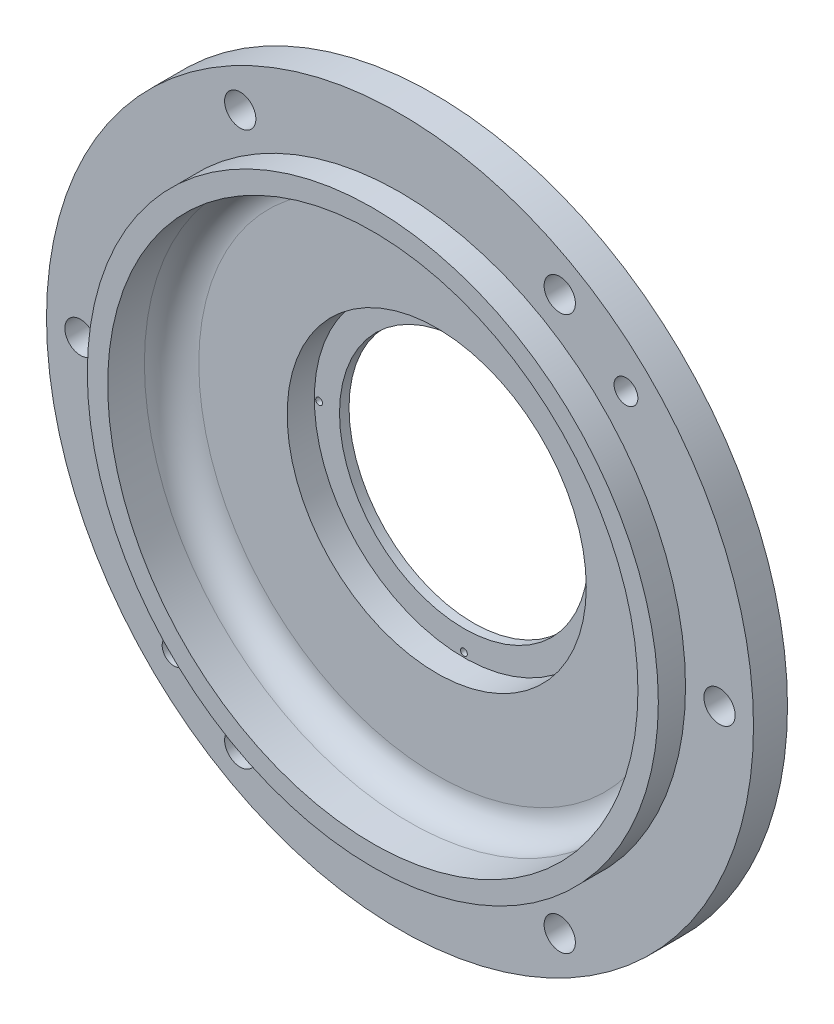
from build123d import *

# Parameters (mm, degrees)
FILLET1_R          = 20
CUT_EXTRUDE1_REACH = 377.068
SKETCH2_R          = 2.5
CIRPATTERN1_COUNT  = 4
CUT_EXTRUDE2_START = -372.639610375
SKETCH3_R          = 11.5
CUT_EXTRUDE2_DEPTH = 377.639610375
CIRPATTERN2_COUNT  = 6
M20_TAPPED_HOLE1_D = 17.5
CIRPATTERN3_COUNT  = 2


with BuildPart() as part:
    # Sketch1 → Revolve1 (revolve)
    with BuildSketch(Plane(origin=(0, 0, 0), x_dir=(0, 0, -1), z_dir=(1, 0, 0)), mode=Mode.PRIVATE) as revolve1_sk:
        Polygon((0, 260), (25, 260), (25, 210), (29.751288694, 210), (54, 168), (54, 91.5), (47, 91.5), (47, 110), (27, 110), (27, 195), (-20, 195), (-20, 210), (0, 210), align=None)
    revolve(revolve1_sk.sketch.rotate(Axis((0, 0, 141.233138436), (0, 0, -1)), 90), axis=Axis((0, 0, 141.233138436), (0, 0, -1)))

    # Fillet1
    fillet1_edges = [part.edges().sort_by_distance(p)[0] for p in [
        (-195, 0, -27),
    ]]
    fillet(fillet1_edges, radius=FILLET1_R)

    # Sketch2 → Cut-Extrude1 (cut, up to next)
    with BuildSketch(Plane(origin=(0, 0, -54), x_dir=(-1, 0, 0), z_dir=(0, 0, -1)), mode=Mode.PRIVATE) as cut_extrude1_sk1:
        with Locations((0, 106.5)):
            Circle(SKETCH2_R)
    cut_extrude1_tool1 = extrude(cut_extrude1_sk1.sketch, amount=-CUT_EXTRUDE1_REACH, mode=Mode.PRIVATE) & part.part
    cut_extrude1 = cut_extrude1_tool1.solids().sort_by_distance((0, 106.5, -54))[0]
    add(cut_extrude1, mode=Mode.SUBTRACT)

    # CirPattern1: Cut-Extrude1 ×4 about axis
    cirpattern1_axis = Axis((0, 0, 0), (0, 0, 1))
    for i in range(1, CIRPATTERN1_COUNT):
        add(cut_extrude1.rotate(cirpattern1_axis, i * 360 / CIRPATTERN1_COUNT), mode=Mode.SUBTRACT)

    # Sketch3 → Cut-Extrude2 (cut)
    with BuildSketch(Plane.XY.offset(CUT_EXTRUDE2_START)):
        with Locations(Location((-235, 0, 0), (0, 0, 180))):
            Circle(SKETCH3_R)
    cut_extrude2 = extrude(amount=CUT_EXTRUDE2_DEPTH, mode=Mode.SUBTRACT)

    # CirPattern2: Cut-Extrude2 ×6 about axis
    cirpattern2_axis = Axis((0, 0, 0), (0, 0, 1))
    for i in range(1, CIRPATTERN2_COUNT):
        add(cut_extrude2.rotate(cirpattern2_axis, i * 360 / CIRPATTERN2_COUNT), mode=Mode.SUBTRACT)

    # M20 Tapped Hole1 (through all)
    with Locations(Plane.XY):
        with Locations((-166.170093579, -166.170093579)):
            m20_tapped_hole1 = Hole(M20_TAPPED_HOLE1_D / 2)

    # CirPattern3: M20 Tapped Hole1 ×2 about axis
    cirpattern3_axis = Axis((0, 0, 0), (0, 0, 1))
    for i in range(1, CIRPATTERN3_COUNT):
        add(m20_tapped_hole1.rotate(cirpattern3_axis, i * 360 / CIRPATTERN3_COUNT), mode=Mode.SUBTRACT)

    # Sketch6 → 1/4 Rc Tapped Hole1 (revolve, cut)
    with BuildSketch(Plane(origin=(0, 187.745212251, -42.600096392), x_dir=(0, 0.8660254037844378, 0.5000000000000014), z_dir=(1, 0, 0))):
        Polygon((0, 0), (0, 278.08587988), (5.35, 278.08587988), (5.35, 11), (5.379117168, 11), (5.7225, 0), align=None)
    revolve(axis=Axis((0, 190.920212251, -48.099357706), (-1.8069730093789398e-15, -0.5000000000000014, 0.8660254037844378)), mode=Mode.SUBTRACT)


solid = part.part
